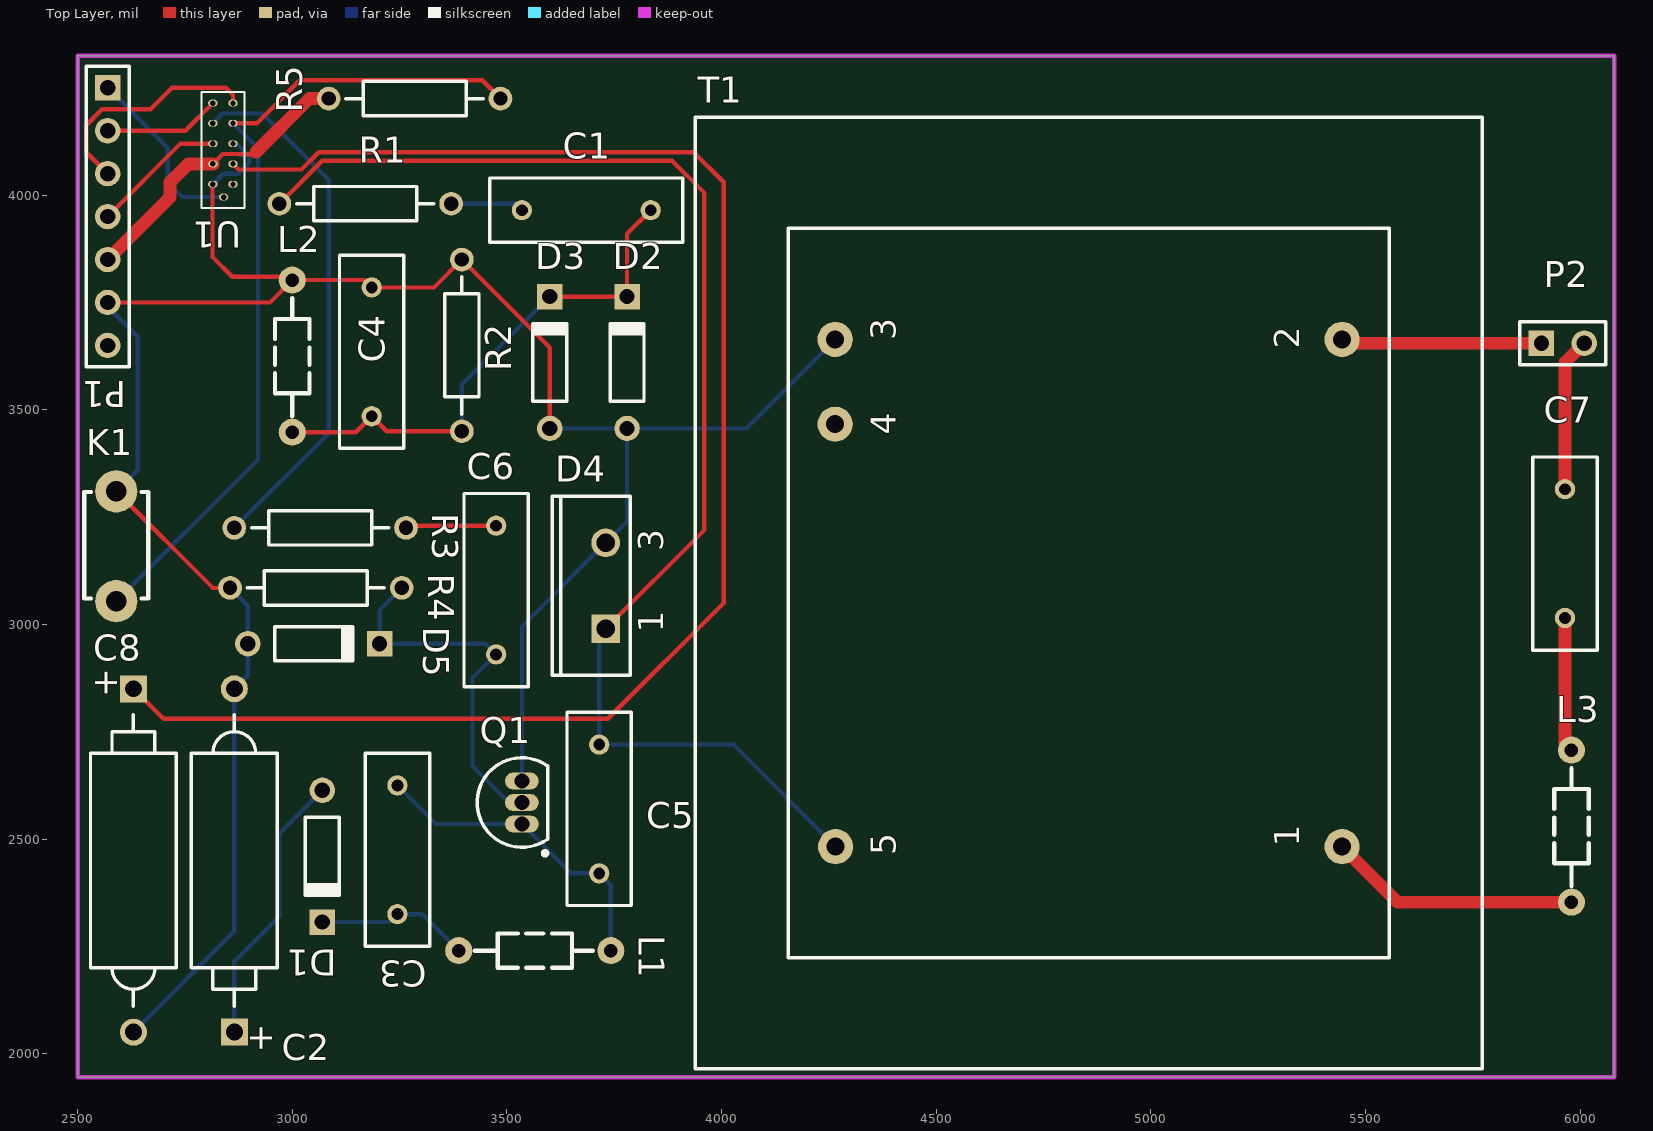
[diagram p0: Top Layer view]
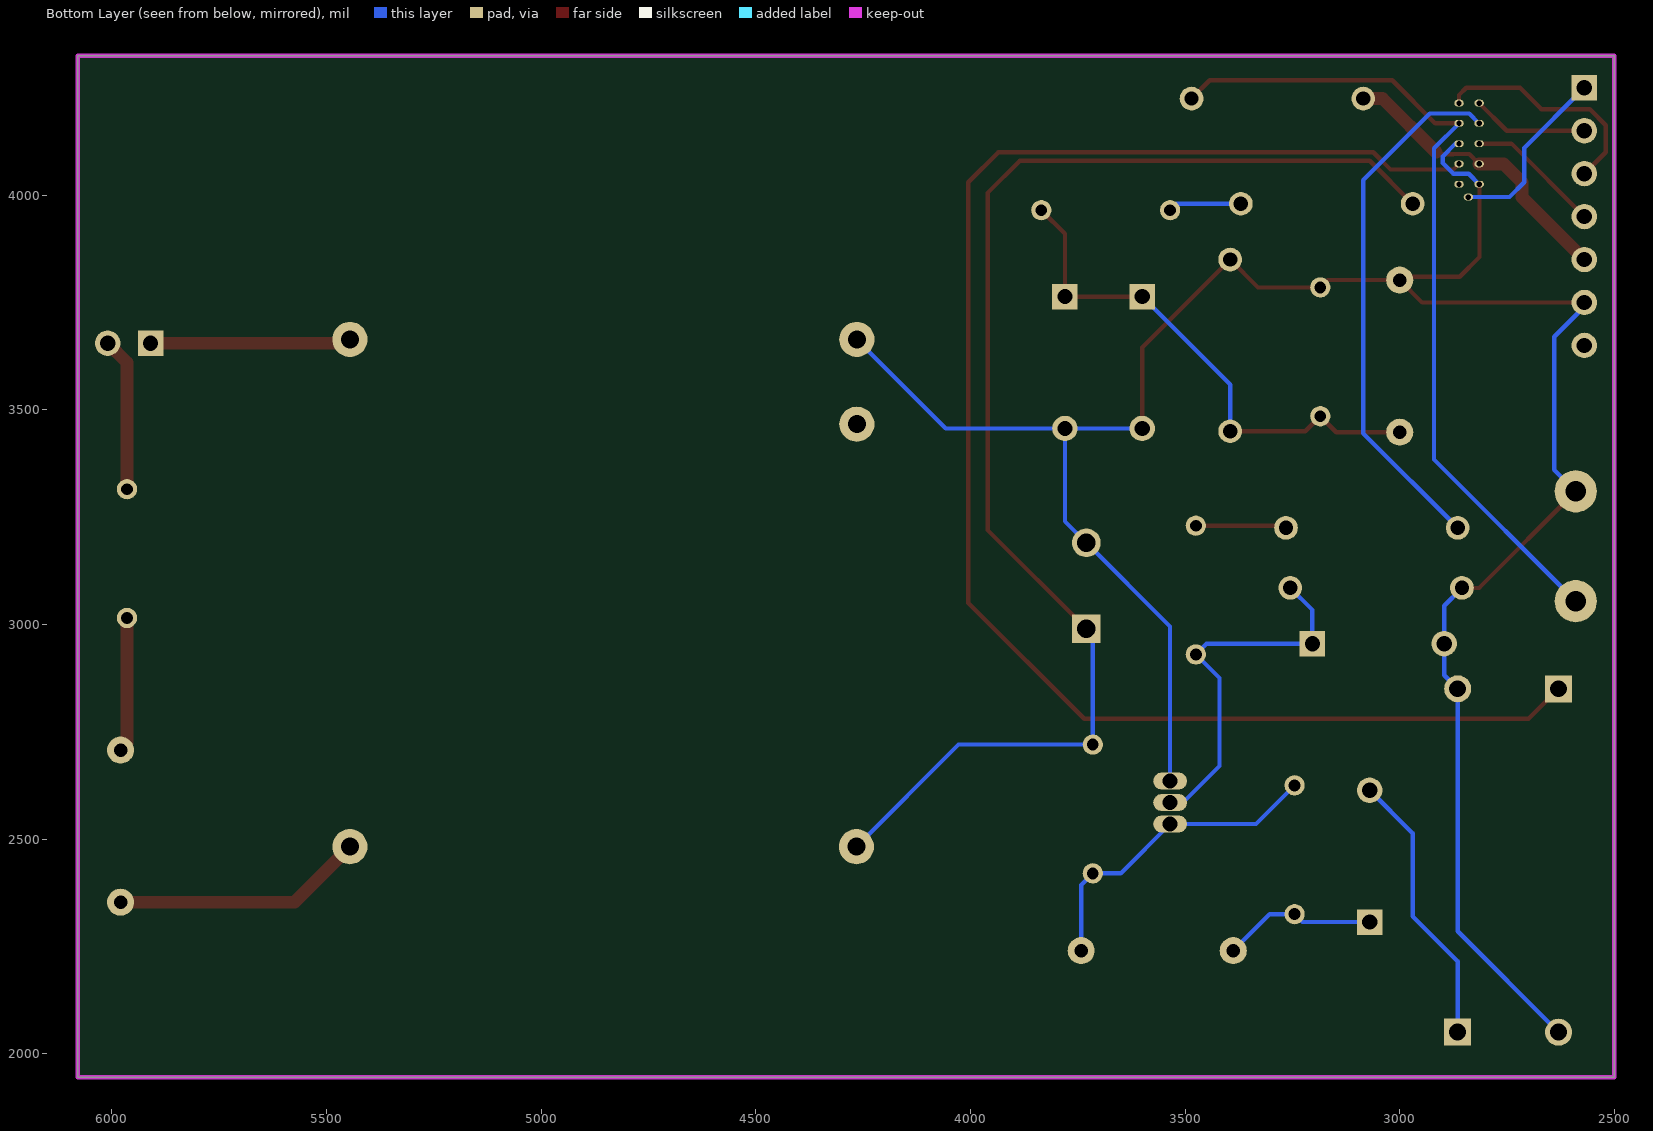
[diagram p1: Bottom Layer view, seen from below]
# Altium PCB MISC76200.PcbDoc
Units mil, origin at the board's own origin, x right, y up, seen from the top; angles counter-clockwise.
Board outline 3580 x 2380 mil, 2 copper layers (Top Layer, Bottom Layer); 27 components, 22 nets, 72 pads, 0 vias.

## Layer stack, top to bottom (the 12.6 mil dielectric is the usual default, probably not edited)
Top Solder: solder mask 0.4, Solder Resist, Dk 3.5
Top Layer: signal copper 1.4
Dielectric 1: dielectric 12.6, FR-4, Dk 4.8
Bottom Layer: signal copper 1.4
Bottom Solder: solder mask 0.4, Solder Resist, Dk 3.5

## Board outline
2500,1945 6080,1945 6080,4325 2500,4325

## Design rules (kind name [scope] priority, off if disabled: settings)
Clearance [All] p1: gap=10
PolygonConnect [All] p1: connectstyle=Relief reliefconductorwidth=10 reliefentries=4 polygonreliefangle="90 Angle" airgapwidth=10
RoutingVias [All] p1: holewidth=28 width=50 viastyle="Through Hole" minholewidth=28 minwidth=50 maxholewidth=28 maxwidth=50
SolderMaskExpansion [All] p1: expansion=4
Width [All] p1: maxlimit=1900 minlimit=10 preferedwidth=10 toplayer_maxwidth=1000 minimp=50.000000 maximp=50.000000 favimp=50.000000
30 further rules are at their usual default settings.

## Components (designator, comment, footprint, x,y, rotation, side; value= is the part's Value field where it differs from the comment)
C1 "1500P" RAD-0.3 3685,3965 r180 top
C2 "100UF/16V" POLAR0.8 2865,2450 r270 top
C3 "0.039UF/50V" RAD-0.3 3245,2475 r270 top
C4 "4700P" RAD-0.3 3185,3635 r90 top
C5 "0.033UF/50V" RAD-0.3 3715,2570 r270 top
C6 "0.33U" RAD-0.3 3475,3080 r90 top
C7 "0.1UF/250V" RAD-0.3 5965,3165 r270 top
C8 "470UF" POLAR0.8 2630,2450 r90 top
D1 "IN5819" DO-35A 3070,2460 r270 top
D2 "IN4148" DO-35A 3780,3610 r90 top
D3 "IN4148" DO-35A 3600,3610 r90 top
D4 "Diode 10TQ040" TO-220AC 3730,3090 r90 top
D5 "IN4148" DO-35A 3050,2955 r0 top
K1 "KEY" DIP-3X6X4.3 2590,3054.09 r90 top
L1 "68UH" AL0204 3565,2240 r0 top
L2 "220UH" AL0204 3000,3625 r90 top
L3 "15UH" AL0204 5980,2530 r90 top
P1 "CON7" HDR1X7 2570,4250 r270 top
P2 "CON2" HDR1X2 5910,3655 r0 top
Q1 "BD139" TO-226-AA 3535,2585 r0 top
R1 "270" AXIAL-0.4 3170,3980 r0 top
R2 "2.7K" AXIAL-0.4 3395,3650 r270 top
R3 "27" AXIAL-0.4 3065,3225 r0 top
R4 "27" AXIAL-0.4 3055,3085 r0 top
R5 "51K" AXIAL-0.4 3285,4225 r180 top
T1 "Trans CT" TRF_5 4855.25,3073 r90 top
U1 "KQ-330K" 20130-10PIN 2838.42,4120 r180 top

## Footprints (in the part's own frame and the unit in brackets; to place one, negate y for a bottom-side part, rotate by r counter-clockwise, add the part's x,y. Pads: shape width x height; smd on the part's side, far side on the other; paste and mask are expansions set on the pad)
20130-10PIN [mm]
  oval 0.56x0.4 hole 0.32 paste+0 mask+0.102: 1(-0.595,2.4) 2(0.595,2.4) 3(-0.595,1.2) 4(0.595,1.2) 5(-0.595,0) 6(0.595,0) 7(-0.595,-1.2) 8(0.595,-1.2) 9(-0.595,-2.4) 10(0.595,-2.4) 11(-0.04,3.162)
  silkscreen extent -1.27,-3.05 1.27,3.81
AL0204 [mm] "9*2*4mm（脚距，直径，长度）"
  round 1.6 hole 0.8: 1(-4.5,0) 2(4.5,0)
  silkscreen extent -3.56,-1.02 3.43,1.02, body extent -4.75,-1.02 4.75,1.02, height 2.07
AXIAL-0.4 [mm] "Axial Device, Thru-Hole; 2 Leads; 0.4 in Pin Spacing"
  round 1.4 hole 0.85: 1(-5.08,0) 2(5.08,0)
  silkscreen extent -4.06,-1.02 4.06,1.02
DIP-3X6X4.3 [mm]
  round 2.5 hole 1.2: 1(0,0) 3(6.5,0)
  silkscreen extent 0.16,-1.9 6.46,1.9, body extent -0.64,-1.75 7.19,1.75, height 4.31
DO-35A [mm] "Diode, Axial; Body 4.6 x 1.9 mm (LxDia. max), Lead Dia. 0.53 mm (max)"
  round 1.5 hole 0.9: 1(-3.9,0)
  rect 1.5x1.5 hole 0.9: 2(3.9,0)
  silkscreen extent -2.3,-1 2.4,1
HDR1X2 [mm] "Connector; Header; 2 Position"
  rect 1.5x1.5 hole 0.9: 1(0,0)
  round 1.5 hole 0.9: 2(2.54,0)
  silkscreen extent -1.27,-1.27 3.81,1.27
HDR1X7 [mm] "Connector; Header; 7 Position"
  rect 1.5x1.5 hole 0.9: 1(0,0)
  round 1.5 hole 0.9: 2(2.54,0) 3(5.08,0) 4(7.62,0) 5(10.16,0) 6(12.7,0) 7(15.24,0)
  silkscreen extent -1.27,-1.27 16.51,1.27
POLAR0.8 [mm] "Polarized Capacitor; 2 Leads"
  rect 1.6x1.6 hole 1: 1(10.16,0)
  round 1.6 hole 1: 2(-10.16,0)
  silkscreen extent -8.64,-2.54 8.64,2.54
RAD-0.3 [mm] "Radial Cap, Thru-Hole; 2 Leads; 0.3 in Pin Spacing"
  round 1.2 hole 0.7: 1(-3.81,0) 2(3.81,0)
  silkscreen extent -5.71,-1.91 5.71,1.91
TO-220AC [mm] "TO, Thru-Hole, Vertical, Heatsink Mounted; 3 In-Line Leads (1 Absent); Pitch 2.54 mm"
  rect 1.7x1.7 hole 1.1: 1(-2.54,0)
  round 1.7 hole 1.1: 3(2.54,0)
  silkscreen extent -5.3,-1.45 5.3,3.15
TO-226-AA [mm] "TO, Flat Index; 3 In-Line, Axial Leads; Body Dia. 4.8mm; Leads 0.55 x 0.51 mm (max)"
  oval 2x1 hole 0.9: 1(0,-1.27) 2(0,0) 3(0,1.27)
  silkscreen extent -2.65,-3.13 1.52,2.65, body extent -2.65,-2.66 1.52,2.66, height 5.33
TRF_5 [mil] "Transformer; 5 Leads"
  round 82 hole 42: 1(-590.83,-590.42) 2(590.83,-590.42) 3(590.83,590.42) 4(393.33,590.42) 5(-590.83,589.58)
  silkscreen extent -1108,-917 1108,916

## Part data
C1 C3 C4 C5 C6 C7: library part Cap, "Capacitor"
C2 C8: library part "Cap Pol2", "Polarized Capacitor (Axial)"
D1 D2 D3 D5: library part "Diode 1N4149", "Computer Diode"
D4: "Schottky Rectifier"
L1 L2 L3: library part INDUCTOR, "INDUCTOR"
P1: library part "Header 7", "Header, 7-Pin"
P2: library part "Header 2", "Header, 2-Pin"
Q1: library part NPN, "NPN Bipolar Transistor"
R1 R2 R3 R4 R5: library part Res2, "Resistor"
T1: "Center-Tapped Transformer (Coupled Inductor Model)"
U1: library part 20130-10PIN

## Nets (pads, with @x,y where several pads share a name; then routed paths per layer and width w, separated by ;. In a path a pad name is that pad's centre, name@x,y a point inside that pad or via, vN(x,y) a via of type N, cw(c..) or ccw(c..) an arc to the next point about the centre after c; other vN are vias at no path point)
5V: P1.5 R5.2 U1.4 | length 691.4
  Top Layer w10: U1.4 2837.88,4095.63 2874.47,4095.63 2875.1,4095 2910,4095 2915,4100
  Top Layer w30: P1.5 2715,3995 2715,4030 2757.76,4072.76 U1.4 ; 2915,4100 3040,4225 R5.2
12V: C2.1 D1.1 | length 648.5
  Bottom Layer w10: C2.1 2865,2215 2970,2320 2970,2513.54 D1.1
G: C2.2 C4.2 C8.2 D2.1 D3.1 D4.3 D5.1 K1.3 L2.2 P1.6 Q1.3 R2.1 R4.1 T1.3 U1.2 U1.5 | length 5592.5
  Top Layer w10: P1.6 2947.83,3750 L2.2 ; K1.3 2815,3085 R4.1 ; U1.2 2813.98,4024.49 2813.98,3856.02 2860,3810 2992.17,3810 L2.2 ; D3.1 3600,3645 R2.1 3330,3785 C4.2 3167.83,3802.17 L2.2
  Bottom Layer w10: P1.6 2570,3740 2640,3670 2640,3360 K1.3 ; C8.2 2865,2285 C2.2 2896.46,2881.46 D5.1 2896.46,3043.54 R4.1 ; U1.2 2839.37,4049.88 2874.47,4049.88 2874.59,4050 2875,4050 2900,4075 2900,4090 2870,4120 U1.5 ; Q1.3 3535,2995 D4.3 3780,3240 D2.1 ; D3.1 D2.1 ; T1.3 4057.46,3456.46 D2.1
NetC1_1: C1.1 C4.1 D2.2 D3.2 L2.1 R2.2 | length 1227.6
  Top Layer w10: L2.1 3147.83,3447.83 C4.1 3220,3450 R2.2 ; D3.2 D2.2 3780,3910 C1.1
  Bottom Layer w10: R2.2 3395,3558.54 D3.2
NetC1_2: C1.2 R1.2 | length 171.2
  Bottom Layer w10: R1.2 3520,3980 C1.2
NetC3_1: C3.1 C5.2 L1.2 Q1.1 | length 746.2
  Bottom Layer w10: C3.1 3335,2535 Q1.1 3650,2420 C5.2 3742.17,2392.83 L1.2
NetC3_2: C3.2 D1.2 L1.1 | length 360.7
  Bottom Layer w10: D1.2 3226.46,2306.46 C3.2 3302.83,2325 L1.1
NetC5_1: C5.1 D4.1 R1.1 T1.5 | length 3098.1
  Top Layer w10: R1.1 3070,4080 3885,4080 3960,4005 3960,3220 D4.1
  Bottom Layer w10: D4.1 3715,2975 C5.1 4027.83,2720 T1.5
NetC6_1: C6.1 D5.2 Q1.2 R4.2 | length 866.1
  Bottom Layer w10: R4.2 3203.54,3033.54 D5.2 3450,2955 C6.1 3420,2875 3420,2670 3505,2585 Q1.2
NetC6_2: C6.2 R3.2 | length 212.1
  Top Layer w10: R3.2 3270,3230 C6.2
NetC7_1: C7.1 P2.2 | length 358.6
  Top Layer w30: C7.1 5965,3610 P2.2
NetC7_2: C7.2 L3.2 | length 314
  Top Layer w30: C7.2 5965,2722.17 L3.2
NetC8_1: C8.1 U1.3 | length 3689.9
  Top Layer w10: C8.1 2700,2780 3735,2780 4005,3050 4005,4030 3935,4100 3061.72,4100 3021.6,4059.88 2874.72,4059.88 U1.3
NetK1_1: K1.1 R5.1 U1.7 | length 1956.3
  Top Layer w10: U1.7 2917.25,4167.25 3017.56,4267.56 3442.44,4267.56 R5.1
  Bottom Layer w10: K1.1 2920,3384.09 2920,4109.09 U1.7
NetL3_1: L3.1 T1.1 | length 587.9
  Top Layer w30: T1.1 5575,2352.83 L3.1
NetP1_1: P1.1 U1.11 | length 436.4
  Top Layer w10: P1.1 P1.1@2580,4260
  Bottom Layer w10: P1.1 2710,4110 2710,4030 2744.49,3995.51 U1.11
NetP1_2: P1.2 U1.10 | length 271.7
  Top Layer w10: P1.2 2750.51,4150 U1.10
NetP1_3: P1.3 U1.9 | length 542.2
  Top Layer w10: P1.3 2520,4100 2520,4162.97 2557.03,4200 2670,4200 2720,4250 2845,4250 2861.84,4233.16 U1.9
  Bottom Layer w10: P1.3 P1.3@2570,4055
NetP1_4: P1.4 U1.6 | length 315.4
  Top Layer w10: P1.4 2740,4120 U1.6
NetP2_1: P2.1 T1.2 | length 468
  Top Layer w30: T1.2 5454.5,3655 P2.1
NetR3_1: R3.1 U1.8 | length 1244.9
  Bottom Layer w10: U1.8 2837.88,4190.12 2874.46,4190.12 2874.58,4190 2930,4190 3085,4035 3085,3445 R3.1
VAA: P1.7
pads on no net: T1.4 U1.1

## Keep-outs
Keep-Out Layer:
  lines w10: 2500,1945 2510,1945 6080,1945 6080,4325 2500,4325 2500,1945